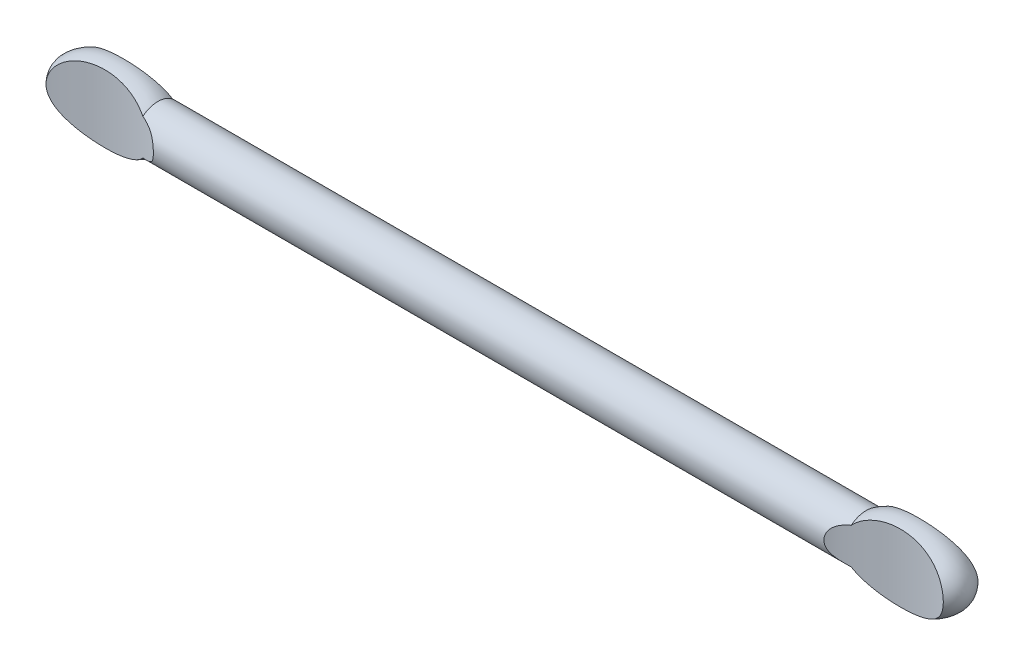
SolidWorks part; units mm, degrees
material "AISI 1045 Steel, cold drawn"
ref_plane "Front Plane" through (0, 0, 0) normal (0, 0, 1) x (1, 0, 0)
ref_plane "Top Plane" through (0, 0, 0) normal (0, 1, 0) x (1, 0, 0)
ref_plane "Right Plane" through (0, 0, 0) normal (1, 0, 0) x (0, 0, -1)
sketch "Sketch1" plane through (0, 0, 0) normal (1, 0, 0) x (0, 0, -1)
  circle A0 centre (0, 0) radius 5
  dimension "D1" = 10
extrude "Boss-Extrude1" add sketch "Sketch1" along normal mid plane 170
sketch "Sketch3" plane through (0, 0, 0) normal (0, 1, 0) x (1, 0, 0)
  line L0 (85, -5) -> (85, 5) construction
  line L1 (-5.5, 0) -> (5.5, 0) construction
  line L2 (85, 0) -> (132.0843, 0) construction
  line L3 (97.5, 0) -> (72.5, 0)
  ellipse E0 centre (85, 0) end of major axis (97.5, 0) minor radius 7.5 (97.5, 0) -> (72.5, 0) ccw
  dimension "D1" = 25
  dimension "D2" = 15
revolve "Revolve3" add sketch "Sketch3" angle 360 about L2
sketch "Sketch4" plane through (0, 0, 0) normal (0, 1, 0) x (1, 0, 0)
  line L0 (106.5078, 0) -> (147.5891, 0) construction
  line L1 (-8.25, 0) -> (8.25, 0) construction
  ellipse E0 centre (85, 7.5) end of major axis (100, 7.5) minor radius 5.5
  ellipse E1 centre (85, 0) end of major axis (97.5, 0) minor radius 7.5 (97.5, 0) -> (75.6831, 5) ccw construction
  ellipse E2 centre (85, -7.5) end of major axis (100, -7.5) minor radius 5.5
  dimension "D1" = 30
  dimension "D2" = 11
extrude "Cut-Extrude1" cut sketch "Sketch4" against normal mid plane 170
mirror "Mirror1" about plane through (0, 0, 0) normal (1, 0, 0) of "Revolve3", "Cut-Extrude1"
